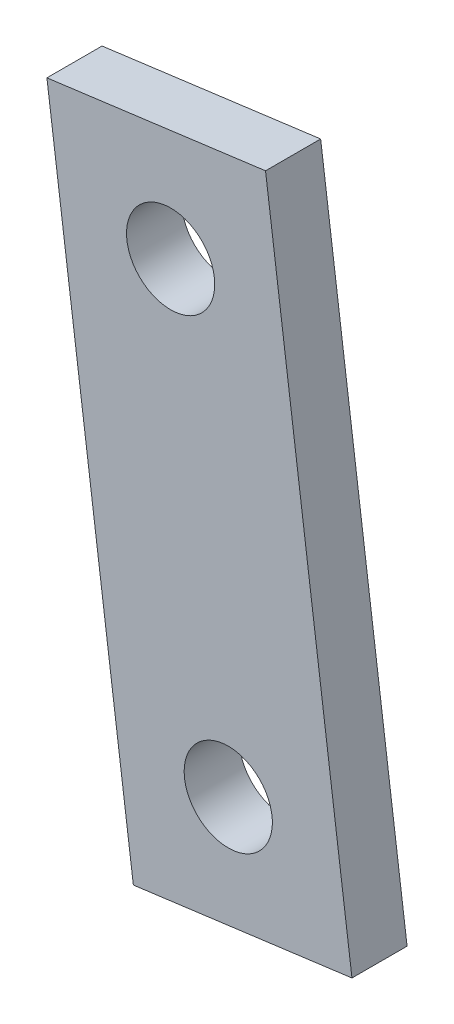
SolidWorks part; units mm, degrees
ref_plane "Front Plane" through (0, 0, 0) normal (0, 0, 1) x (1, 0, 0)
ref_plane "Top Plane" through (0, 0, 0) normal (0, 1, 0) x (1, 0, 0)
ref_plane "Right Plane" through (0, 0, 0) normal (1, 0, 0) x (0, 0, -1)
sketch "Sketch1" plane through (0, 0, 0) normal (0, 0, 1) x (1, 0, 0)
  line L0 (5176.9624, 2249.9426) -> (5189.5263, 2251.5981) construction
  line L1 (5137.3052, 2244.7171) -> (5129.467, 2304.203)
  line L2 (5129.467, 2304.203) -> (5169.1242, 2309.4284)
  line L3 (5169.1242, 2309.4284) -> (5184.8007, 2190.4568)
  line L4 (5184.8007, 2190.4568) -> (5145.1435, 2185.2313)
  line L5 (5145.1435, 2185.2313) -> (5137.3052, 2244.7171)
  circle A0 centre (5151.9084, 2286.9871) radius 8
  circle A1 centre (5162.3593, 2207.6727) radius 8
  dimension "D1" = 40
  dimension "D2" = 40
  dimension "D3" = 120
  dimension "D4" = 20
extrude "Boss-Extrude1" add sketch "Sketch1" along normal blind 10
